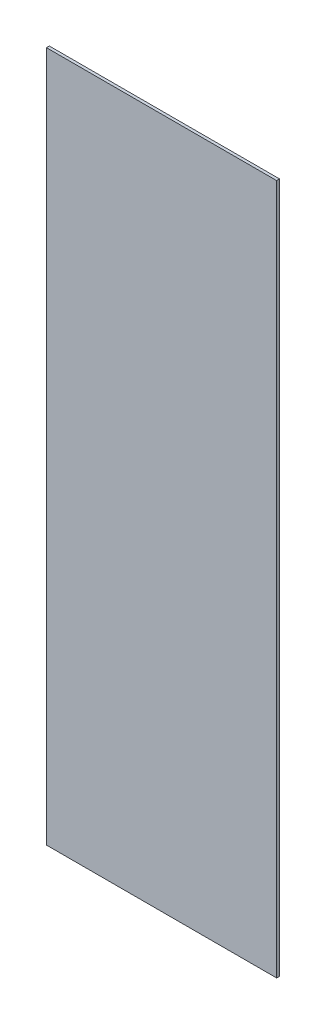
from build123d import *

# Parameters (mm, degrees)
SKETCH1_W           = 80
SKETCH1_H           = 240
BOSS_EXTRUDE1_DEPTH = 1


with BuildPart() as part:
    # Sketch1 → Boss-Extrude1 (new body)
    with BuildSketch(Plane.XY):
        Rectangle(SKETCH1_W, SKETCH1_H)
    extrude(amount=BOSS_EXTRUDE1_DEPTH)


solid = part.part
